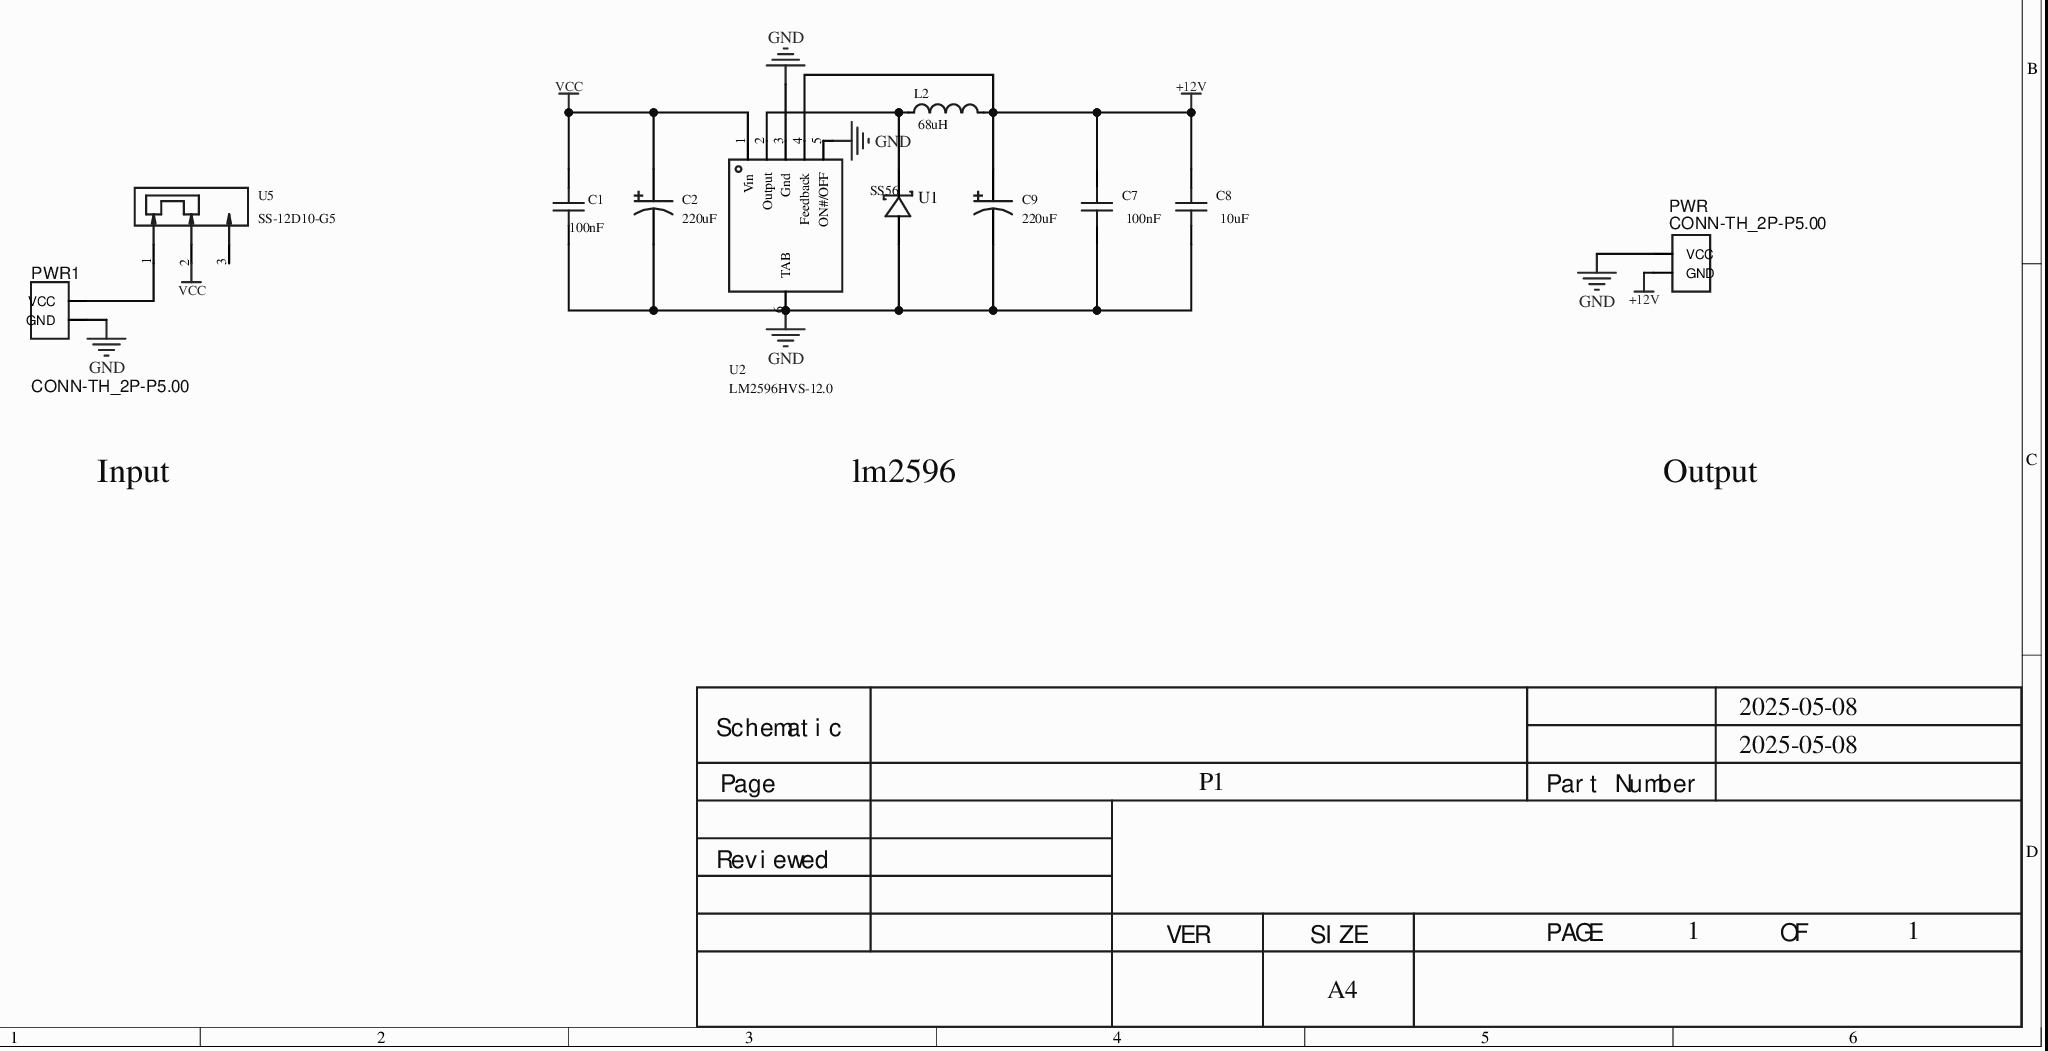
[diagram p0: MISC49950-3.schdoc]
# Altium project MISC49950-2.PrjPcb
1 sheet, 11 parts. Net scope: global (net labels, ports and power ports of the same name join across sheets).
Board file: MISC49950.pcbdoc

## Sheet MISC49950-3.schdoc
size 297 x 210 mm; Version: V1.0; @Project Name: MISC49950; @Page Count: 1; @Update Date: 2025-05-08; @Create Date: 2025-05-08; @Schematic Name: MISC49950; @Page No: 1; @Board Name: MISC49950; @Create Time: 15:52:23; @Update Time: 15:52:31

### Parts
C1  100nF  [C1206]
C2  220uF  [CAP-SMD_BD10.0-L10.3-W10.3-FD-LS11.3]
C7  100nF  [C1206]
C8  10uF  [C0805]
C9  220uF  [CAP-SMD_BD8.0-L8.3-W8.3-FD-1]
L2  68uH  [IND-SMD_L12.0-W12.0_744771008]
PWR  CONN-TH_2P-P5.00  [CONN-TH_2P-P5.00]
PWR1  CONN-TH_2P-P5.00  [CONN-TH_2P-P5.00]
U1  SS56  [SMC_L6.9-W5.9-LS7.9-RD]
U2  LM2596HVS-12.0  [TO-263-5_L10.0-W8.4-P1.70-LS15.3-BR]
U5  SS-12D10-G5  [SW-TH_SS-12D10-G050]

### Nets
+12V: C7.2 C8.2 C9.1 L2.2 PWR.2(GND) U2.4(Feedback)
GND: C1.1 C2.2 C7.1 C8.1 C9.2 PWR.1(VCC) PWR1.2(GND) U1.2(A) U2.3(Gnd) U2.5(ON#/OFF) U2.6(TAB)
VCC: C1.2 C2.1 U2.1(Vin) U5.2
NetL2_1: L2.1 U1.1(C) U2.2(Output)
NetPWR1_1: PWR1.1(VCC) U5.1

Not connected (* = marked no-connect by the designer): U5 3*

### Notes on the sheet
- Input
- lm2596
- Output
- 2025-05-08
- Schematic
- Page
- P1
- Part Number
- Reviewed
- VER
- SIZE
- A4
- PAGE
- 1
- OF

### Library data of the parts
C1 = CAP_0603: ConvertToPcb: yes; SymbolName: CapAcitance; ModelId: ac125912035d415993ca9572d50418b1; ModelName: C0603_L1.6-W0.8-H0.8; ModelTransform: 62.992,31.496,0,0,0,0,0,0,0; Device: CAP_0603; AddInBom: yes; Supplier Footprint: 0603; FootprintName: C1206; Value: 100nF
C2 C9 = VEJ222M1ATR-1313: Capacitance:2200uF;Tolerance:±20%;Rated voltage:10V;Body diameter:12.5mm;Body length:13.5mm;Ripple current:-;ESR:-;Life:2000hrs@105℃;Operating temperature:-45℃~+105℃;; Manufacturer: lelon(立隆); Symbol: VEJ222M1A1313-TRO; AddInBom: yes; ModelId: 6392bc9430a7457794798829c6f11371; ModelName: CAP-SMD_BD12.5-L13.0-W13.0-LS13.7-FD; ModelTransform: 539.369,511.81,0,180,0,0,0,0,0; Tolerance: ±20%; Rated Voltage: 10V; φD: 12.5mm; L: 13.5mm; Value: 220uF; Device: VEJ222M1ATR-1313; LCSC Part Name: 2200uF ±20% 10V; SupplierPart: C249623; ManufacturerPart: VEJ222M1ATR-1313; Supplier Footprint: SMD,D12.5xL13.5mm; JLCPCB Part Class: Extended library; Datasheet: https://atta.szlcsc.com/upload/public/pdf/source/20181120/C249623_15A2F235CA4672A97EC0D1FDEBBD7E7E.pdf; Supplier: LCSC; ConvertToPcb: yes; Ripple Current: -; Equivalent Series Resistance(ESR): -; Lifetime @ Temp: 2000hrs@105℃; Operating Temperature: -45℃~+105℃
  C2: FootprintName: CAP-SMD_BD10.0-L10.3-W10.3-FD-LS11.3
  C9: FootprintName: CAP-SMD_BD8.0-L8.3-W8.3-FD-1
C7 = CAP_1206: ConvertToPcb: yes; SymbolName: CapAcitance; ModelId: c6790e9475e1483991d2c64340b24e96; ModelName: C1206_L3.2-W1.6-H1.3; ModelTransform: 125.984,62.992,0,0,0,0,0,0,0; Device: CAP_1206; AddInBom: yes; Supplier Footprint: 1206; FootprintName: C1206; Value: 100nF
C8 = CAP_0805: ConvertToPcb: yes; SymbolName: CapAcitance; ModelId: 1ba041120af144c991958decab20d241; ModelName: C0805_L2.0-W1.3-H1.3; ModelTransform: 78.74,51.181,0,0,0,0,0,0.0005,0; Value: 10uF; Device: CAP_0805; AddInBom: yes; Supplier Footprint: 0805; FootprintName: C0805
L2 = L_0603: Symbol: SDFL1608S100KTF; AddInBom: yes; ModelId: 2bc5ec593d464d6ba9807aec0b5673c2; ModelName: L0603_L1.6-W0.8-H0.5_BEAD; ModelTransform: 63,31.5,19.7,0,0,0,0,0,0; Value: 68uH; Device: L_0603; Supplier Footprint: L0603; ConvertToPcb: yes; FootprintName: IND-SMD_L12.0-W12.0_744771008
PWR PWR1 = CONN-TH_2P-P5.00: Convert to PCB: yes; Origin Footprint: CONN-TH_2P-P5.00; Device: CONN-TH_2P-P5.00; Symbol: CONN-TH_2P-P5.00; Add into BOM: yes; Supplier: LCSC; FootprintName: CONN-TH_2P-P5.00
U1 = SS56_C2931905: DC reverse voltage (Vr):60V;Average rectified current (Io):5A;Forward voltage (Vf):700mV@5A;Reverse current (Ir):1mA@60V;; Manufacturer: Doeshare(德芯); Symbol: SBD; Voltage - DC Reverse (Vr) (Max): 60V; Current - Average Rectified (Io): 5A; Diode Configuration: Single; AddInBom: yes; ModelId: 4f14ab132b494223bc17c7f39616ac35; ModelTransform: 314.96,236.22,0,0,0,0,0,0,0; Device: SS56_C2931905; Voltage - Forward (Vf) (Max) @ If: 700mV @ 5A; Value: SS56; Type: Diode; LCSC Part Name: 60V 5A 700mV@5A; Supplier Part: C2931905; Supplier: LCSC; Reverse Voltage (Vr): 60V; Average Rectified Current (Io): 5A; Forward Voltage (Vf@If): 700mV@5A; Reverse Leakage Current (Ir): 1mA@60V; ManufacturerPart: SS56; Supplier Footprint: SMC; JLCPCB Part Class: Extended Part; Datasheet: https://atta.szlcsc.com/upload/public/pdf/source/20220113/189652AD5D386E8C0BF30073E8292F53.pdf; ConvertToPcb: yes; FootprintName: SMC_L6.9-W5.9-LS7.9-RD; ModelName: SMC_L6.9-W5.9-LS7.9-RD
U2 = LM2596HVS-5.0: Manufacturer: UMW(广东友台半导体); Symbol: LM2596HVS-5.0_C347445; AddInBom: yes; ModelId: fb036f748a274327bb376552b66e43ac; ModelTransform: 388.9756,661.416,0,90,0,0,-43.311,0,0; Manufacturer Part: LM2596HVS-12.0; Device: LM2596HVS-5.0; LCSC Part Name: LM2596HVS-5.0; SupplierPart: C347445; Supplier Footprint: TO-263-5; JLCPCB Part Class: Extended library; Datasheet: https://atta.szlcsc.com/upload/public/pdf/source/20211011/C7416AEF3194BD283261B8F2553C4145.pdf; Supplier: LCSC; ConvertToPcb: yes; FootprintName: TO-263-5_L10.0-W8.4-P1.70-LS15.3-BR; ModelName: TO-263-5_L10.0-W8.4-P1.70-LS15.3-BR
U5 = SS-12D10-G5: Manufacturer: DEALON(德艺隆); AddInBom: yes; ModelId: 15e778c65cea4653be5d87f0502c04df; ModelTransform: 499.999,263.779,0,0,0,0,0,0,-196.85; Device: SS-12D10-G5; Symbol: SS-12D10-G5; LCSC Part Name: 插件大电流拨动开关; SupplierPart: C2998777; ManufacturerPart: SS-12D10-G5; Supplier Footprint: 插件; JLCPCB Part Class: Extended library; Datasheet: https://atta.szlcsc.com/upload/public/pdf/source/20220428/E10CB334ACBAF32CF4AF8D87DA871CD3.pdf; Supplier: LCSC; ConvertToPcb: yes; FootprintName: SW-TH_SS-12D10-G050; ModelName: SW-TH_SS-12D10-G050